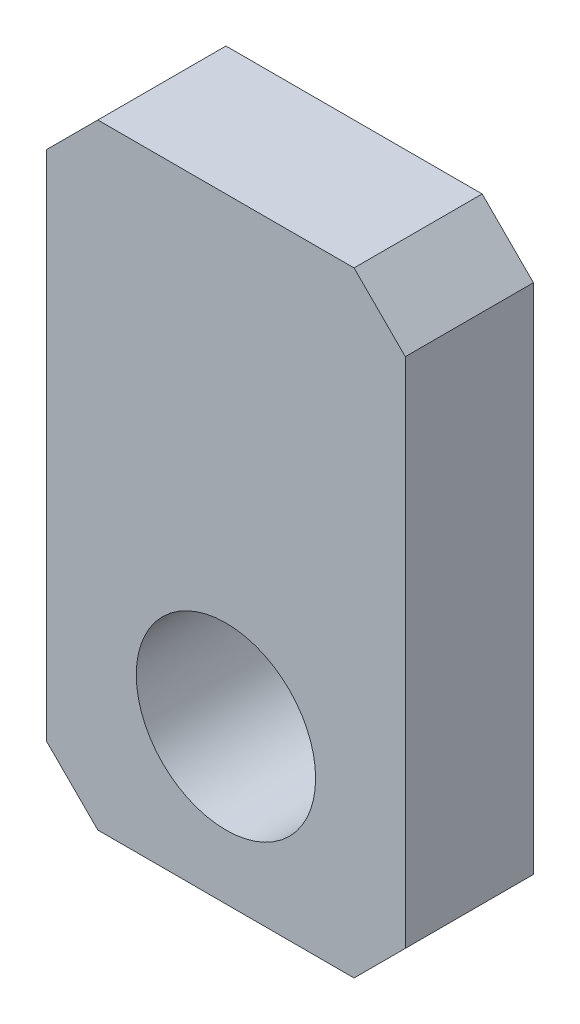
from build123d import *

# Parameters (mm, degrees)
SKETCH1_W                  = 7
SKETCH1_H                  = 12
BOSS_EXTRUDE1_DEPTH        = 1.25
F_3_5_3_5_DIAMETER_HOLE1_D = 3.5
CHAMFER1_SIZE              = 1


with BuildPart() as part:
    # Sketch1 → Boss-Extrude1 (new, symmetric)
    with BuildSketch(Plane.XY):
        Rectangle(SKETCH1_W, SKETCH1_H)
    extrude(amount=BOSS_EXTRUDE1_DEPTH, both=True)

    # Ø3.5 (3.5) Diameter Hole1 (through all)
    with Locations(Plane.XY.offset(1.25)):
        with Locations((0, -3)):
            Hole(F_3_5_3_5_DIAMETER_HOLE1_D / 2)

    # Chamfer1
    chamfer1_edges = [part.edges().sort_by_distance(p)[0] for p in [
        (3.5, -6, 0),
        (-3.5, -6, 0),
        (-3.5, 6, 0),
        (3.5, 6, 0),
    ]]
    chamfer(chamfer1_edges, length=CHAMFER1_SIZE)


solid = part.part
